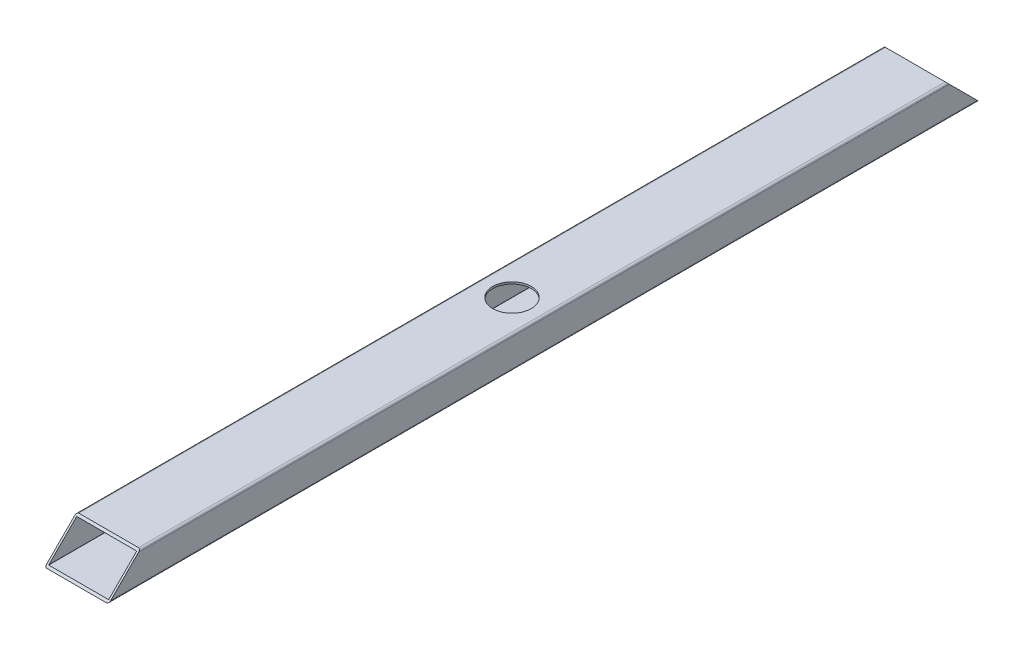
from build123d import *

# Parameters (mm, degrees)
EXTRUDE_1_DEPTH     = 1400
CUT_EXTRUDE_1_DEPTH = 1400
SKETCH_3_R          = 30.15
CUT_EXTRUDE_2_DEPTH = 218


with BuildPart() as part:
    # 草图1 → 凸台-拉伸1 (new body)
    with BuildSketch(Plane.XY):
        with BuildLine():
            Line((-46.8, 25), (46.8, 25))
            ThreePointArc((46.8, 25), (49.0627417, 24.0627417), (50, 21.8))
            Line((50, 21.8), (50, -21.8))
            ThreePointArc((50, -21.8), (49.0627417, -24.0627417), (46.8, -25))
            Line((46.8, -25), (-46.8, -25))
            ThreePointArc((-46.8, -25), (-49.0627417, -24.0627417), (-50, -21.8))
            Line((-50, -21.8), (-50, 21.8))
            ThreePointArc((-50, 21.8), (-49.0627417, 24.0627417), (-46.8, 25))
        make_face()
        with BuildLine():
            Line((-46.8, 22), (46.8, 22))
            ThreePointArc((46.8, 22), (46.941421356, 21.941421356), (47, 21.8))
            Line((47, 21.8), (47, -21.8))
            ThreePointArc((47, -21.8), (46.941421356, -21.941421356), (46.8, -22))
            Line((46.8, -22), (-46.8, -22))
            ThreePointArc((-46.8, -22), (-46.941421356, -21.941421356), (-47, -21.8))
            Line((-47, -21.8), (-47, 21.8))
            ThreePointArc((-47, 21.8), (-46.941421356, 21.941421356), (-46.8, 22))
        make_face(mode=Mode.SUBTRACT)
    extrude(amount=EXTRUDE_1_DEPTH)

    # 草图2 → 切除-拉伸1 (cut)
    with BuildSketch(Plane(origin=(50, 0, 0), x_dir=(0, 0, -1), z_dir=(1, 0, 0))):
        Polygon((-1318.410144038, 25), (-1368.410144038, -25), (-1510.151659449, -71.563080947), (-1552.75637803, 36.507424721), align=None)
        Polygon((-54.410144038, 25), (-4.410144038, -25), (36.992690616, -46.405998122), (74.054919354, -20.164122041), (119.219041394, 25), (0, 63.525051138), align=None)
    extrude(amount=-CUT_EXTRUDE_1_DEPTH, mode=Mode.SUBTRACT)

    # 草图3 → 切除-拉伸2 (cut)
    with BuildSketch(Plane(origin=(0, 25, 0), x_dir=(1, 0, 0), z_dir=(0, 1, 0))):
        with Locations(Location((0, -686.410144038, 0), (0, 0, 270))):
            Circle(SKETCH_3_R)
    extrude(amount=-CUT_EXTRUDE_2_DEPTH, mode=Mode.SUBTRACT)


solid = part.part
